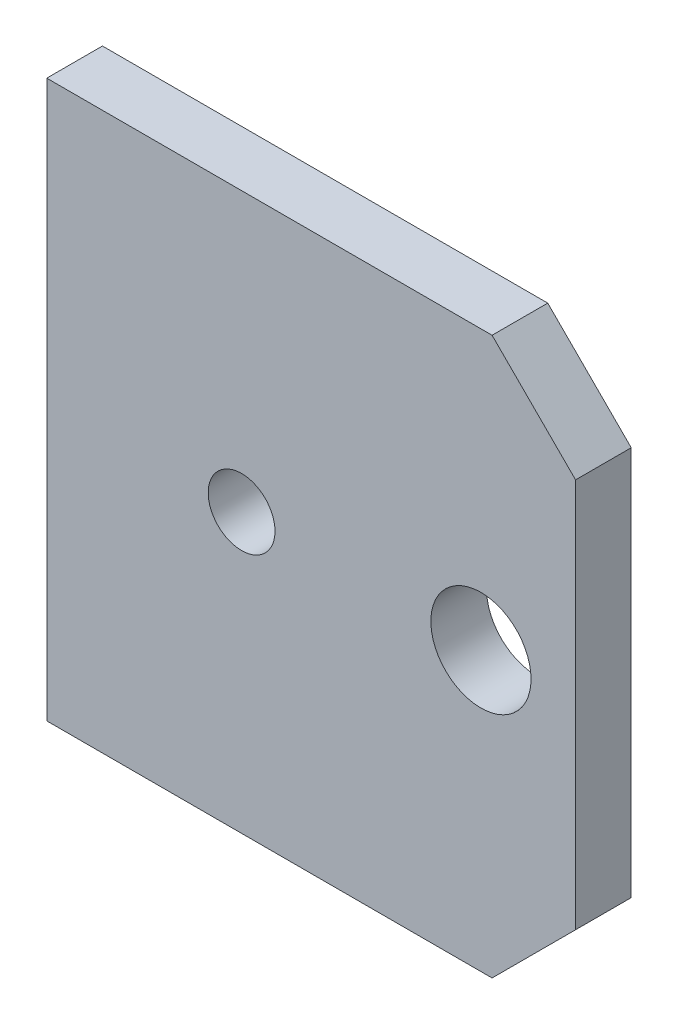
SolidWorks part; units mm, degrees
material "1023 碳钢板 (SS)"
ref_plane "前视基准面" through (0, 0, 0) normal (0, 0, 1) x (1, 0, 0)
ref_plane "上视基准面" through (0, 0, 0) normal (0, 1, 0) x (1, 0, 0)
ref_plane "右视基准面" through (0, 0, 0) normal (1, 0, 0) x (0, 0, -1)
sketch "草图1" plane through (0, 0, 0) normal (0, 0, 1) x (1, 0, 0)
  line L0 (47.5, 35) -> (32.5, 50)
  line L1 (32.5, 50) -> (-47.5, 50)
  line L2 (47.5, 35) -> (47.5, -35)
  line L3 (32.5, -50) -> (-47.5, -50)
  line L4 (-47.5, 50) -> (-47.5, -50)
  line L5 (47.5, 50) -> (-47.5, -50) construction
  line L6 (47.5, -50) -> (-47.5, 50) construction
  line L7 (47.5, -35) -> (32.5, -50)
  circle A0 centre (-12.5, 0) radius 6
  circle A1 centre (30.5, 0) radius 9
  point P0 (0, 0)
  dimension "D3" = 18
  dimension "D4" = 12
  dimension "D5" = 43
  dimension "D1" = 95
  dimension "D2" = 100
  dimension "D6" = 17
extrude "凸台-拉伸1" add sketch "草图1" along normal blind 10
